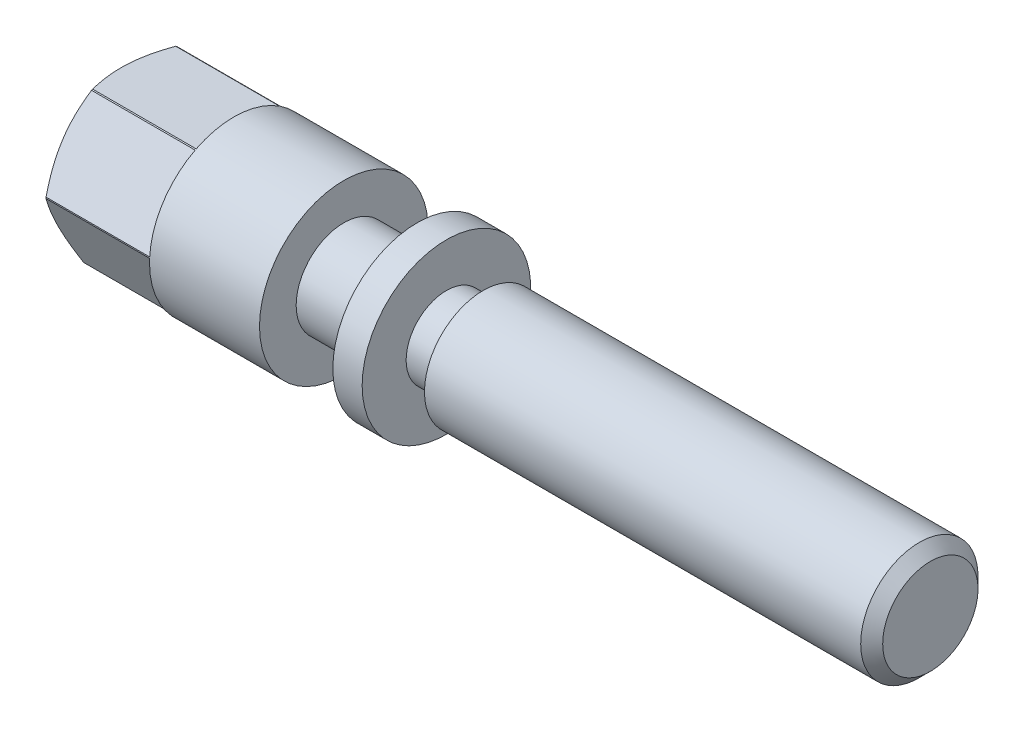
from build123d import *

# Parameters (mm, degrees)
M12_TAPPED_HOLE1_D           = 10.2
M12_TAPPED_HOLE1_DEPTH       = 23.25
M12_TAPPED_HOLE1_CSINK_D     = 12.05
M12_TAPPED_HOLE1_CSINK_ANGLE = 90
M12_TAPPED_HOLE1_TIP         = 3.064389157
SKETCH4_R                    = 21.574990141
CUT_EXTRUDE1_DEPTH           = 15
CHAMFER1_SIZE                = 1.5


with BuildPart() as part:
    # Sketch1 → Revolve1 (revolve)
    with BuildSketch(Plane.XY, mode=Mode.PRIVATE) as revolve1_sk:
        Polygon((0, 0), (0, 10), (0.866025404, 11.5), (30, 11.5), (30, 6.5), (40, 6.5), (40, 11.5), (44, 11.5), (44, 5.5), (49, 5.5), (49, 8), (110, 8), (110, 0), align=None)
    revolve(revolve1_sk.sketch.rotate(Axis((0, 0, 0), (1, 0, 0)), 90), axis=Axis((0, 0, 0), (1, 0, 0)))

    # M12 Tapped Hole1
    with Locations(Plane(origin=(0, 0, 0), x_dir=(0, 0, -1), z_dir=(-1, 0, 0))):
        with Locations((0, 0)):
            CounterSinkHole(M12_TAPPED_HOLE1_D / 2, M12_TAPPED_HOLE1_CSINK_D / 2, depth=M12_TAPPED_HOLE1_DEPTH, counter_sink_angle=M12_TAPPED_HOLE1_CSINK_ANGLE)
            with Locations((0, 0, -(M12_TAPPED_HOLE1_DEPTH + M12_TAPPED_HOLE1_TIP / 2))):  # 118° drill point
                Cone(0, M12_TAPPED_HOLE1_D / 2, M12_TAPPED_HOLE1_TIP, mode=Mode.SUBTRACT)

    # Sketch4 → Cut-Extrude1 (cut)
    with BuildSketch(Plane.ZY):
        Circle(SKETCH4_R)
        Polygon((5.227352222, 10.296024576), (-6.30294273, 9.675032107), (-11.530294952, -0.620992469), (-5.227352222, -10.296024576), (6.30294273, -9.675032107), (11.530294952, 0.620992469), align=None, mode=Mode.SUBTRACT)
    extrude(amount=-CUT_EXTRUDE1_DEPTH, mode=Mode.SUBTRACT)

    # Chamfer1
    chamfer1_edges = [part.edges().sort_by_distance(p)[0] for p in [
        (110, 0, -8),
    ]]
    chamfer(chamfer1_edges, length=CHAMFER1_SIZE)


solid = part.part
